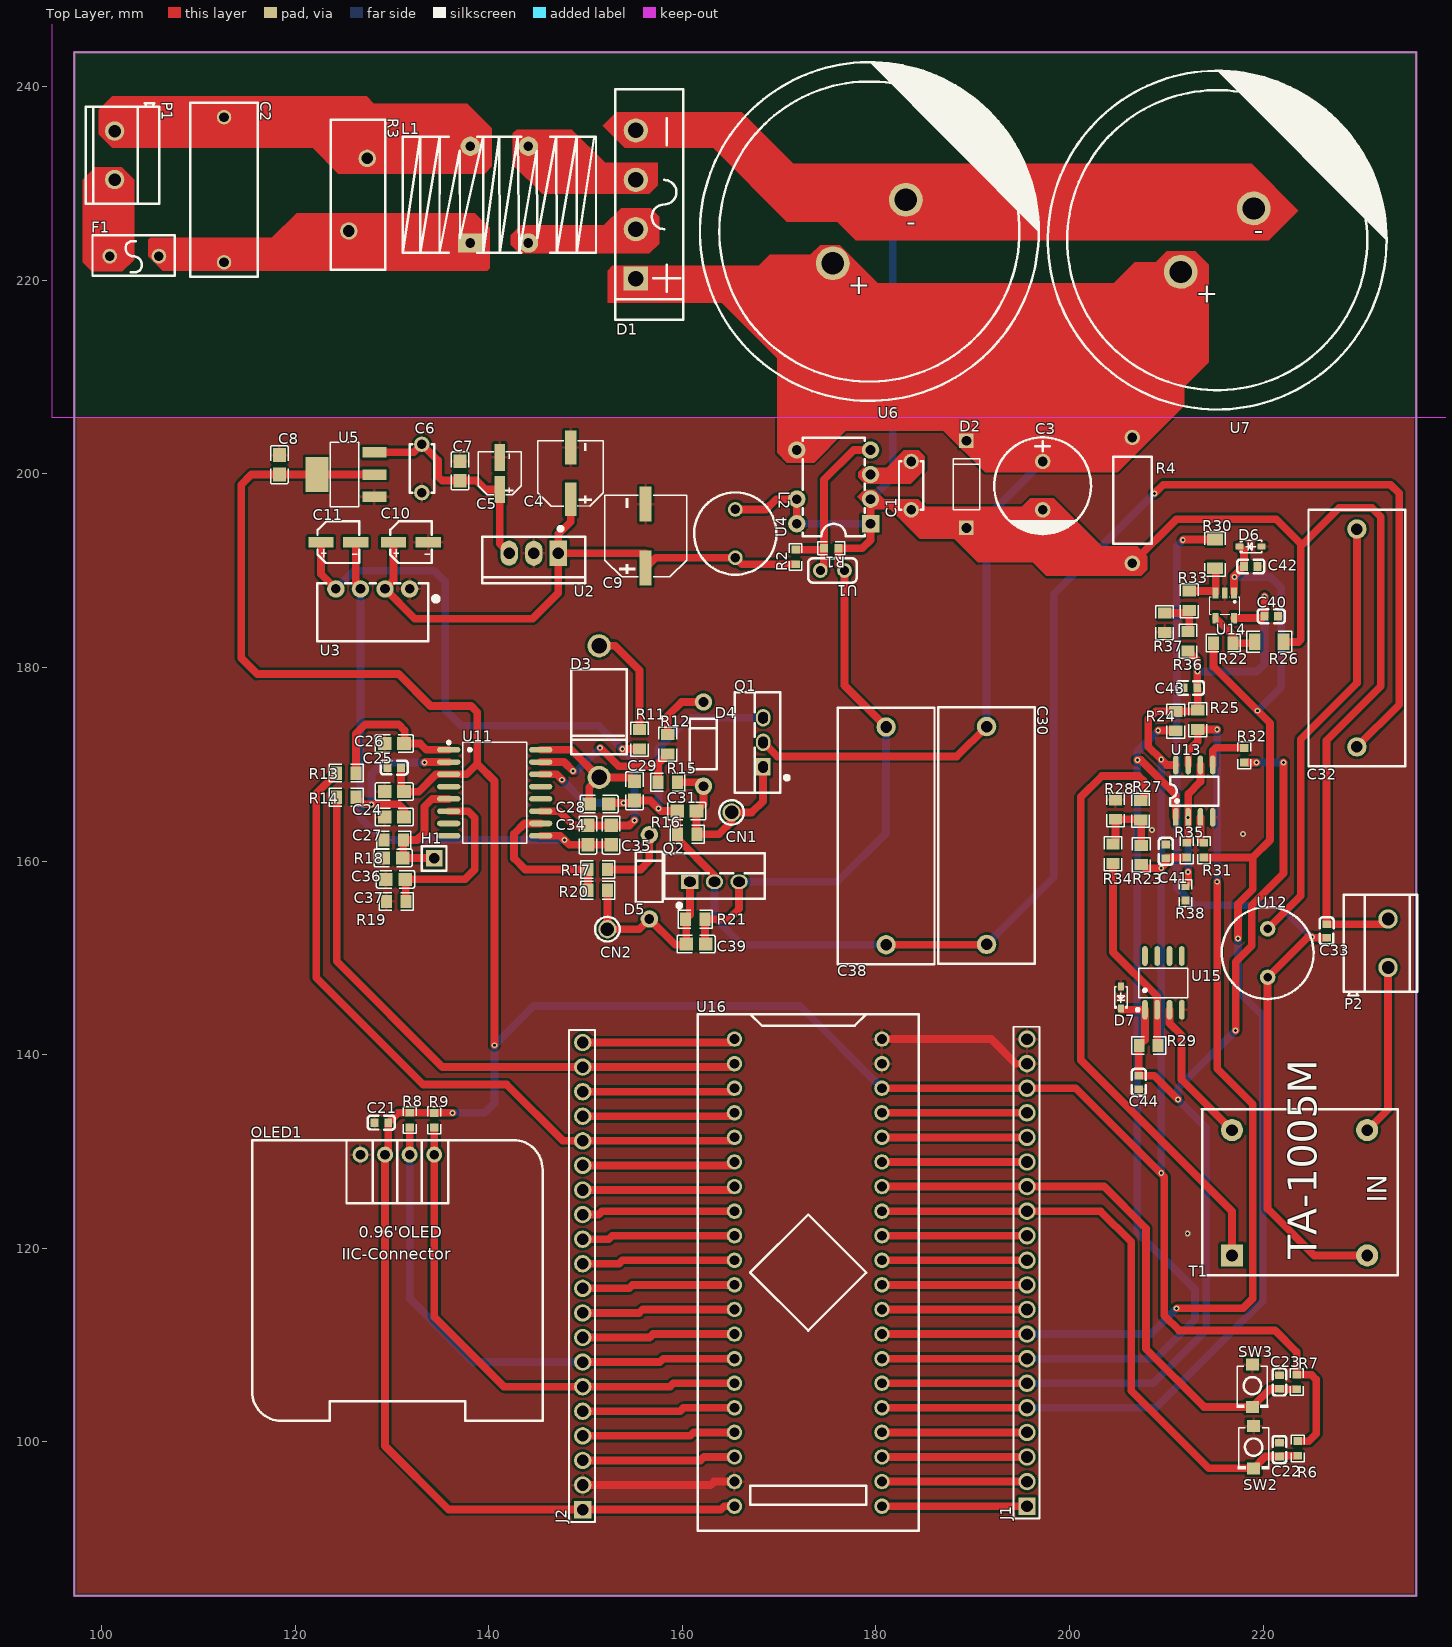
[diagram p0: Top Layer view]
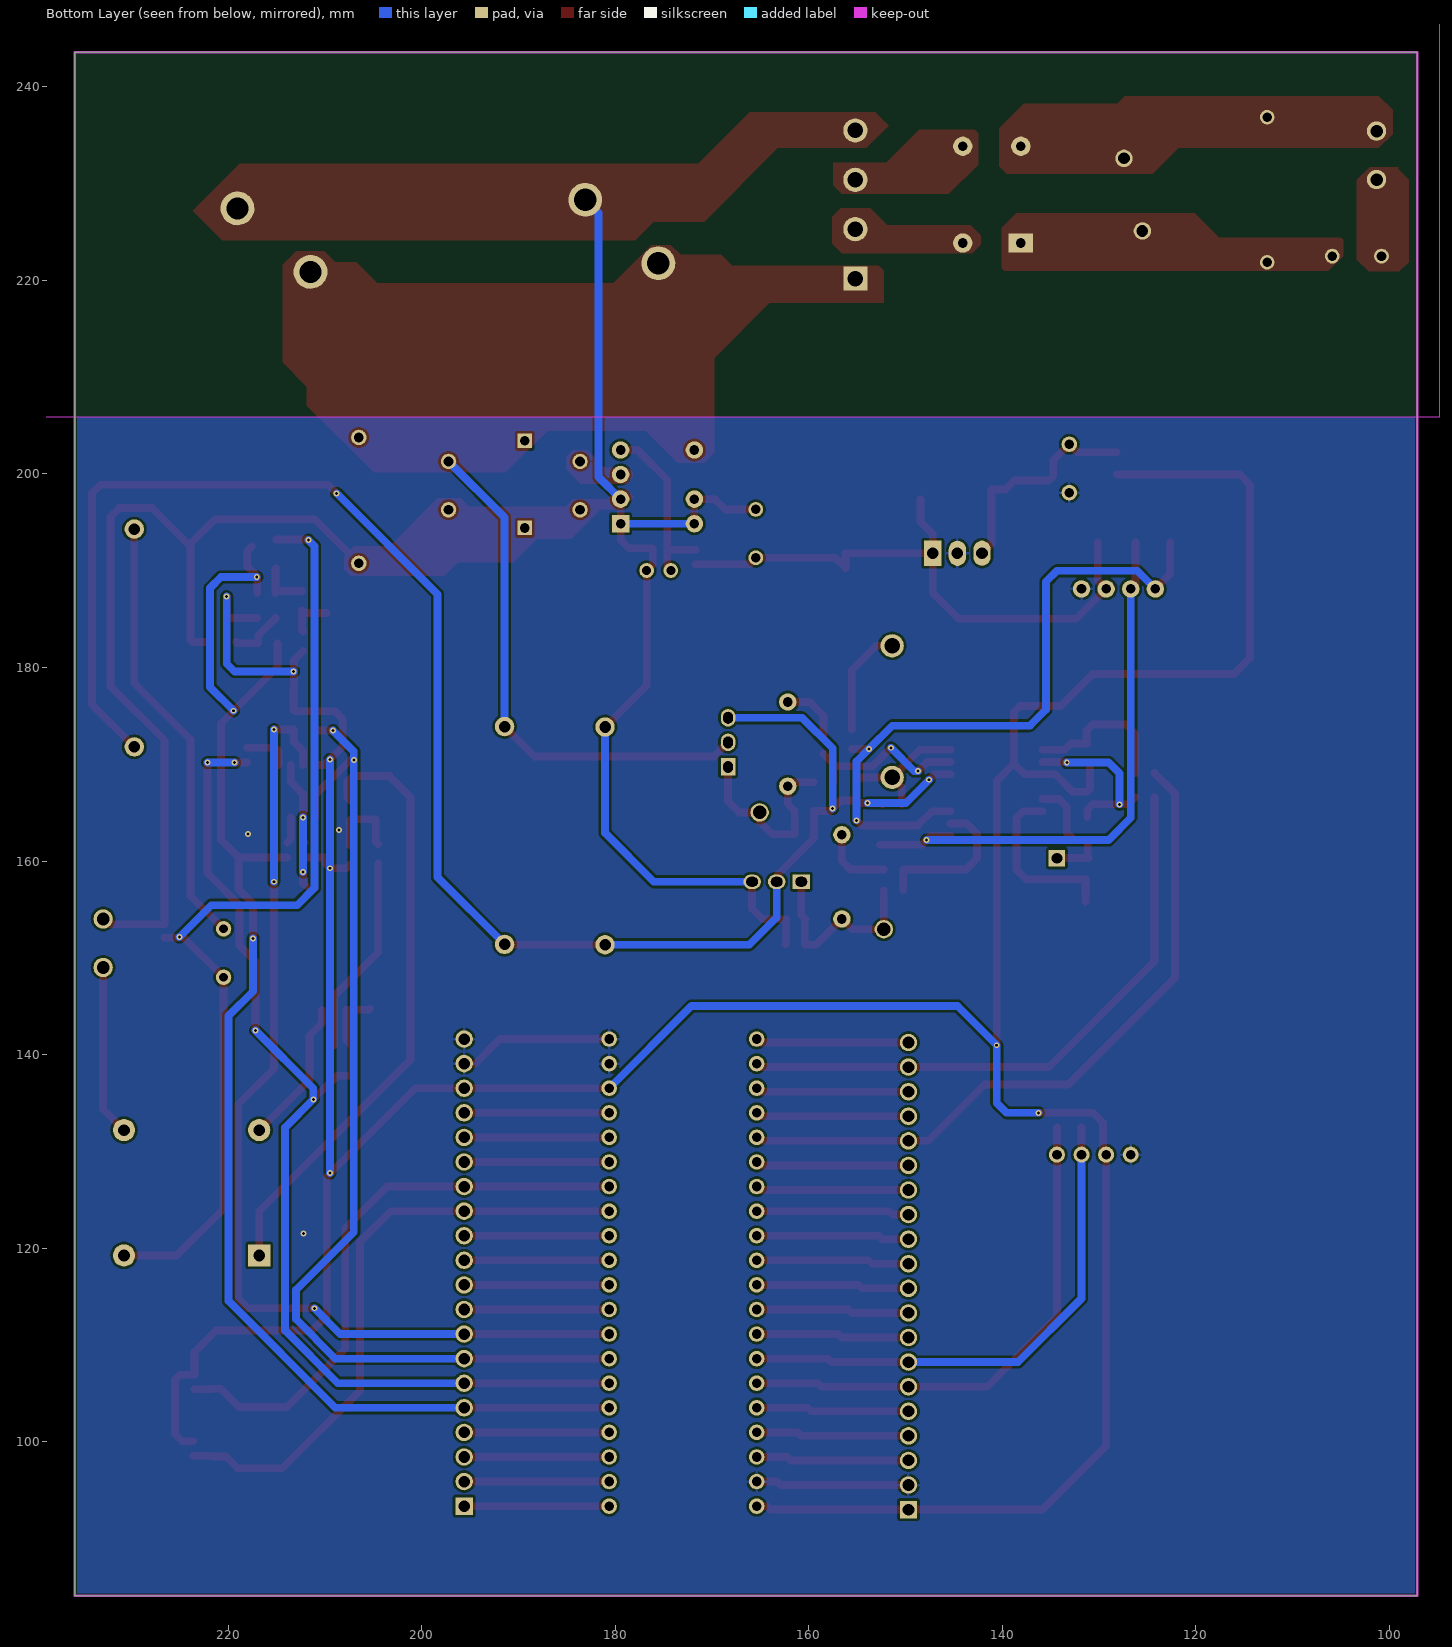
[diagram p1: Bottom Layer view, seen from below]
# Altium PCB MISC51807.pcbdoc
Units mm, origin at the board's own origin, x right, y up, seen from the top; angles counter-clockwise.
Board outline 138.68 x 159.51 mm, 2 copper layers (Top Layer, Bottom Layer), stack 1.58 mm thick; 107 components, 77 nets, 334 pads, 37 vias.

## Layer stack, top to bottom
Top Solder Mask Layer: solder mask 0.01, Dk 3.3
Top Layer: signal copper 0.035
Dielectric1: surface 1.51, FR4, Dk 4.5
Bottom Layer: signal copper 0.035
Bottom Solder Mask Layer: solder mask 0.01, Dk 3.3

## Board outline
97.155,243.586 97.155,84.074 235.839,84.074 235.839,243.586

## Design rules (kind name [scope] priority, off if disabled: settings)
BoardOutlineClearance copperThickness2oz_1 [All] p2 off: genericclearance=0.203 ignorepadtopadclearanceinfootprint=FALSE except(0: Arc-SplitContinuation Track-SplitContinuation SMDPad-SplitContinuation THPad-SplitContinuation Via-SplitContinuation Fill-SplitContinuation Region-SplitContinuation Poly-SplitContinuation Text-SplitContinuation Hole-SplitContinuation; 0.152: Arc-CutoutEdge SMDPad-CutoutEdge THPad-CutoutEdge Via-CutoutEdge Fill-CutoutEdge Region-CutoutEdge Text-CutoutEdge; 0.176: Hole-OutlineEdge Hole-CutoutEdge; 0.254: Poly-OutlineEdge Poly-CutoutEdge; 0.3: Arc-OutlineEdge Track-OutlineEdge SMDPad-OutlineEdge THPad-OutlineEdge Via-OutlineEdge Fill-OutlineEdge Region-OutlineEdge Text-OutlineEdge Track-CutoutEdge)
BoardOutlineClearance copperThickness1oz_1 [All] p4: genericclearance=0.102 ignorepadtopadclearanceinfootprint=FALSE except(0: Arc-SplitContinuation Track-SplitContinuation SMDPad-SplitContinuation THPad-SplitContinuation Via-SplitContinuation Fill-SplitContinuation Region-SplitContinuation Poly-SplitContinuation Text-SplitContinuation Hole-SplitContinuation; 0.152: SMDPad-CutoutEdge THPad-CutoutEdge Via-CutoutEdge Fill-CutoutEdge Region-CutoutEdge Text-CutoutEdge; 0.176: Hole-OutlineEdge Hole-CutoutEdge; 0.254: Poly-OutlineEdge Poly-CutoutEdge; 0.3: Arc-OutlineEdge Track-OutlineEdge SMDPad-OutlineEdge THPad-OutlineEdge Via-OutlineEdge Fill-OutlineEdge Region-OutlineEdge Text-OutlineEdge Arc-CutoutEdge Track-CutoutEdge)
Clearance copperThickness2oz [All] p1 off: gap=0.203 ignorepadtopadclearanceinfootprint=FALSE except(0.152: SMDPad-Track SMDPad-SMDPad THPad-Track SMDPad-THPad THPad-THPad Track-Via SMDPad-Via THPad-Via Via-Via Fill-Track Region-Track Fill-SMDPad Region-SMDPad Fill-THPad Region-THPad Fill-Via Region-Via Fill-Fill Fill-Region Region-Region Arc-Track Arc-SMDPad Arc-THPad Arc-Via Fill-Arc Region-Arc Arc-Arc Text-Track SMDPad-Text Text-THPad Text-Via Fill-Text Region-Text Arc-Text Text-Text; 0.176: Hole-Track Hole-SMDPad Hole-THPad Hole-Via Fill-Hole Region-Hole Hole-Arc Hole-Text; 0.254: Poly-Track Poly-SMDPad Poly-THPad Poly-Via Poly-Fill Poly-Region Poly-Poly Poly-Arc Poly-Text Poly-Hole)
Clearance copperThickness1oz [All] p3: gap=0.102 ignorepadtopadclearanceinfootprint=FALSE except(0.152: SMDPad-Track SMDPad-SMDPad THPad-Track SMDPad-THPad THPad-THPad Track-Via SMDPad-Via THPad-Via Via-Via Fill-Track Region-Track Fill-SMDPad Region-SMDPad Fill-THPad Region-THPad Fill-Via Region-Via Fill-Fill Fill-Region Region-Region Arc-Track Arc-SMDPad Arc-THPad Arc-Via Fill-Arc Region-Arc Arc-Arc Text-Track SMDPad-Text Text-THPad Text-Via Fill-Text Region-Text Arc-Text Text-Text; 0.176: Hole-Track Hole-SMDPad Hole-THPad Hole-Via Fill-Hole Region-Hole Hole-Arc Hole-Text; 0.254: Poly-Track Poly-SMDPad Poly-THPad Poly-Via Poly-Fill Poly-Region Poly-Poly Poly-Arc Poly-Text Poly-Hole)
DiffPairsRouting differentialPair [All] p1: maxlimit=0.152 minlimit=0.152 mostfreqgap=0.152 toplayer_minwidth=0.127 toplayer_prefwidth=0.254 toplayer_maxwidth=2.54 toplayer_mingap=0.152 toplayer_prefgap=0.152 toplayer_maxgap=0.152 bottomlayer_minwidth=0.127 bottomlayer_prefwidth=0.254 bottomlayer_maxwidth=2.54 bottomlayer_mingap=0.152 bottomlayer_prefgap=0.152 bottomlayer_maxgap=0.152 maxuncoupledlength=0.254
HoleToHoleClearance otherClearance [All] p1: gap=0.3 allowstackedmicrovias=TRUE
Length netLength [All] p1: minlimit=0 maxlimit=0
MatchedLengths netLengthTolerance [All] p1: tolerance=25.4
PasteMaskExpansion pasteMaskExpansion [All] p1: expansion=0
PlaneConnect innerPlane [All] p1: planeconnectstyle=Relief reliefexpansion=0.508 reliefentries=4 reliefconductorwidth=0.254 reliefairgap=0.254
PolygonConnect copperRegion [(InNet('GND'))] p1: connectstyle=Relief reliefconductorwidth=0.254 reliefentries=4 polygonreliefangle="90 Angle" airgapwidth=0.254 via.connectstyle=Relief via.reliefconductorwidth=0.254 via.reliefentries=4 via.polygonreliefangle="90 Angle" via.airgapwidth=0.254
RoutingVias viaSize [All] p1: holewidth=0.305 width=0.61 viastyle="Through Hole" minholewidth=0.3 minwidth=0.5 maxholewidth=6.3 maxwidth=10
SolderMaskExpansion solderMaskExpansion [IsVia] p1: expansion=-25.4 istentingtop=TRUE
SolderMaskExpansion solderMaskExpansion [All] p2: expansion=0.051 istentingtop=FALSE
Width copperThickness2oz_2 [All] p1 off: maxlimit=2.54 minlimit=0.203 preferedwidth=0.254
Width copperThickness1oz_2 [All] p2: maxlimit=2.54 minlimit=0.127 preferedwidth=0.254

## Components (designator, comment, footprint, x,y, rotation, side; value= is the part's Value field where it differs from the comment)
C1 "100nF" CAP-TH_L5.0-W2.5-P5.00-D1.0 183.639,198.789 r90 top
C2 "330nF" CAP-TH_L18.0-W7.0-P15.00-D0.7 112.649,229.362 r270 top
C3 "10uF" CAP-TH_BD10.0-P5.00-D0.6-FD_1 197.228,198.789 r270 top
C4 "100uF" CAP-SMD_BD6.3-L6.6-W6.6-FD 148.46,200.059 r90 top
C5 "10uF" CAP-SMD_BD4.0-L4.3-W4.3-FD 141.13,200.044 r90 top
C6 "100nF" CAP-TH_L5.0-W2.5-P5.00-D1.0 133.093,200.567 r90 top
C7 "10uF" C0805 137.03,200.313 r270 top
C8 "10uF" C0805 118.361,200.948 r270 top
C9 "470uF" CAP-SMD_BD8.0-L8.3-W8.3-LS9.2-FD-H10.5 156.207,193.582 r90 top
C10 "10uF" CAP-SMD_BD4.0-L4.3-W4.3-FD_1 131.95,192.947 r0 top
C11 "10uF" CAP-SMD_BD4.0-L4.3-W4.3-FD_1 124.457,192.947 r0 top
C21 "100nF" C0603 128.905,132.969 r0 top
C22 "100nF" C0603 221.692,99.187 r270 top
C23 "100nF" C0603 221.692,106.172 r270 top
C24 "10uF" C0805 130.238,167.171 r0 top
C25 "100nF" C0603 130.245,169.652 r0 top
C26 "22PF" C0805 130.238,172.137 r180 top
C27 "22PF" C0805 130.238,164.548 r0 top
C28 "100nf" C0805 151.395,165.883 r0 top
C29 "2.2uf" C0805 155.067,167.259 r270 top
C30 "10uF/630V CBB" "1uf/630V CBB" 191.389,162.687 r270 top
C31 "1nf" C0805 160.463,165.162 r0 top
C32 "10uF/630V CBB" "1uf/630V CBB" 229.743,183.007 r90 top
C33 "100nF" C0603 226.568,152.781 r270 top
C34 "100nF" C0805 150.241,162.687 r270 top
C35 "2.2uf" C0805 152.654,162.687 r270 top
C36 "22pf" C0805 130.111,160.326 r0 top
C37 "100nF" C0805 130.365,158.115 r0 top
C38 "10uF/630V CBB" "1uf/630V CBB" 181.102,162.56 r90 top
C39 "1nf" C0805 161.415,151.421 r180 top
C40 "100nF" C0603 220.853,185.293 r0 top
C41 "100nF" C0603 209.955,161.004 r90 top
C42 "100nF" C0603 218.726,190.442 r180 top
C43 "100nF" C0603 212.495,177.895 r180 top
C44 "100nF" C0603 207.161,137.128 r270 top
CN1 "RH-5001" TEST-TH_BD2.54-P1.4_BLACK 165.083,165.025 r0 top
CN2 "RH-5001" TEST-TH_BD2.54-P1.4_BLACK 152.256,152.96 r0 top
D1 "KBU810" DIO-BG-TH_L23.2-W6.8-P5.10_KBU 155.194,227.838 r270 top
D2 "BYV26C" DO-41_BD2.6-L5.1-P9.00-D0.8-RD 189.354,198.916 r270 top
D3 "SR5100" DO-201AD_BD5.3-L8.4-P12.50-D1.4-RD 151.395,175.439 r90 top
D4 "1N5819" DO-41_BD2.4-L4.7-P8.70-D0.9-FD 162.179,172.085 r90 top
D5 "1N5819" DO-41_BD2.4-L4.7-P8.70-D0.9-FD 156.591,158.369 r90 top
D6 "BZT52C3V3S" SOD-323_L1.7-W1.3-LS2.6-RD 218.718,192.5 r0 top
D7 "BZT52C3V3S" SOD-323_L1.7-W1.3-LS2.6-RD 205.312,145.894 r90 top
F1 "MTS1315A" FUSE-TH_L8.4-W4.0-P5.08-D0.6 103.378,222.504 r0 top
H1 "PZ254V-11-01P" HDR-TH_1P-P2.54-V-M 134.366,160.274 r0 top
J1 "2.54-1*20P直针" HDR-TH_20P-P2.54-V-M-1 195.612,117.48 r90 top
J2 "2.54-1*20P直针" HDR-TH_20P-P2.54-V-M-1 149.708,117.122 r90 top
L1 "PDMCAT16128-103ML" IND-TH_4P-L20.0-W12.0-P6.00-LS10.0-BL 141.097,228.854 r0 top
L2 "1mH" IND-TH_BD8.5-P5.00-D0.6 165.478,193.836 r270 top
OLED1 "" 0.96OLED_4P 130.556,129.667 r0 top
P1 "CONN-TH_2P-P5.00" CONN-TH_2P-P5.00 101.346,232.918 r270 top
P2 "CONN-TH_2P-P5.00" CONN-TH_2P-P5.00 232.918,151.511 r90 top
Q1 "IRF840" TO-220-3_L10.2-W4.5-P2.54-L-1 168.348,172.264 r90 top
Q2 "IRF840" TO-220-3_L10.2-W4.5-P2.54-L-1 163.322,157.861 r0 top
R1 "6.2kΩ" R0603 175.384,192.312 r180 top
R2 "20kΩ" R0603 171.701,191.423 r90 top
R3 "420pF@1kHz" RES-TH_L15.5-W5.6-P7.50-D0.8-S1.90 126.492,228.854 r270 top
R4 "220kΩ" RES-TH_BD3.9-L9.0-P13.00-D0.8 206.499,197.265 r90 top
R6 "10kΩ" R0603_1 223.597,99.314 r90 top
R7 "10kΩ" R0603_1 223.47,106.172 r90 top
R8 "4.7kΩ" R0603 131.826,133.24 r90 top
R9 "4.7kΩ" R0603 134.366,133.223 r90 top
R11 "4.7R" R0805#1 155.575,172.593 r90 top
R12 "4.7R" R0805#1 158.496,172.085 r90 top
R13 "47R" R0805#1 125.285,169.089 r0 top
R14 "47R" R0805#1 125.285,166.603 r0 top
R15 "10r" R0805#1 158.496,168.148 r180 top
R16 "10K" R0805#1 160.515,162.766 r0 top
R17 "4.7R" R0805#1 151.257,159.131 r0 top
R18 "10K" R0805#1 130.175,162.179 r0 top
R19 "4.7k" R0805#1 130.429,155.829 r0 top
R20 "10r" R0805#1 151.257,156.972 r180 top
R21 "10K" R0805#1 161.341,153.978 r180 top
R22 "10kΩ" R0805#1 215.89,182.518 r180 top
R23 "10kΩ" R0805#1 207.415,160.623 r90 top
R24 "10kΩ" R0805#1 210.971,174.466 r270 top
R25 "10kΩ" R0805#1 213.257,174.593 r270 top
R26 "1MΩ" R1206 220.634,182.645 r180 top
R27 "100Ω" R0805#1 207.352,165.259 r270 top
R28 "10kΩ" R0805#1 204.748,165.322 r90 top
R29 "820Ω" R0805#2 208.177,140.938 r0 top
R30 "1MΩ" R1206 215.035,191.738 r270 top
R31 "1kΩ" R0603 213.892,161.131 r90 top
R32 "1kΩ" R0603 218.059,170.942 r270 top
R33 "10kΩ" R0805#1 212.368,186.912 r90 top
R34 "100Ω" R0805#1 204.494,160.75 r90 top
R35 "100kΩ" R0603 212.114,161.131 r270 top
R36 "10kΩ" R0805#1 212.241,182.721 r270 top
R37 "10kΩ" R0805#1 209.828,184.626 r90 top
R38 "3.3kΩ" R0603_NEW 211.987,156.686 r90 top
SW2 "TS-1088-AR02016" SW-SMD_L3.9-W3.0-P4.45 219.025,99.441 r270 top
SW3 "TS-1088-AR02016" SW-SMD_L3.9-W3.0-P4.45 218.898,105.791 r270 top
T1 "TA-1005M" TA-1005M 216.789,119.253 r90 top
U1 "10nF" CAP-TH_L5.0-W2.5-P2.50-D0.5 175.511,190.026 r180 top
U2 "LM7805" TO-220-3_L10.0-W4.5-P2.54-L 144.65,191.804 r180 top
U3 "260kHz" PWRM-TH_4P-L11.5-W6.0-P2.54_B1503S 128.013,188.121 r180 top
U4 "LNK304PN" DIP-8_7P-L9.7-W6.4-P2.54-LS7.6-BL-PE6 175.638,198.662 r90 top
U5 "AMS1117-3.3" SOT-223-3_L6.5-W3.4-P2.30-LS7.0-BR 125.219,199.932 r0 top
U6 "470uF" CAP-TH_BD35.0-P10.00-D1.5-FD 179.324,225.044 r0 top
U7 "470uF" CAP-TH_BD35.0-P10.00-D1.5-FD 215.265,224.155 r0 top
U11 "UCC21520ADWR" SOIC-16_L10.3-W7.5-P1.27-LS10.3-BL 140.618,167.057 r270 top
U12 "2.5mH" IND-TH_BD9.5-P5.00-D0.7 220.472,150.495 r270 top
U13 "LM393DR" SOIC-8_L5.0-W4.0-P1.27-LS6.0-BL 212.896,167.227 r0 top
U14 "AD8605ARTZ-REEL7" SOT-23-5_L3.0-W1.7-P0.95-LS2.8-BR 216.051,186.404 r90 top
U15 "LM358DT" SOIC-8_L4.9-W3.9-P1.27-LS6.0-BL 209.701,147.415 r0 top
U16 "STM32F103C8T6-Card" CONN-TH_L53.3-W22.9_STM32F103C8T6-CARD 173.006,117.48 r270 top

## Footprints (in the part's own frame and the unit in brackets; to place one, negate y for a bottom-side part, rotate by r counter-clockwise, add the part's x,y. Pads: shape width x height; smd on the part's side, far side on the other; paste and mask are expansions set on the pad)
0.96OLED_4P [mm]
  round 1.65 hole 1 copper offset 0,0: 1(-3.81,-0.001) 2(-1.27,0.002) 3(1.27,0.002) 4(3.81,0.002)
  silkscreen extent -15,-27.5 15,1.5
"1uf/630V CBB" [mm]
  round 2 hole 1.2: 1(-11.208,0.047) 2(11.292,0.047)
  silkscreen extent -13.21,-4.95 13.29,5.05
C0603 [mm]
  rect 0.8x0.9 smd paste+0 mask+0.051: 1(-0.7,0) 2(0.7,0)
  silkscreen extent -1.41,-0.71 1.39,0.72
C0805 [mm]
  rect 1.41x1.35 smd paste-100 mask+0.051: 1(-1,0) 2(1,0)
  silkscreen extent -1.96,-0.9 1.96,0.9
CAP-SMD_BD4.0-L4.3-W4.3-FD [mm]
  rect 2.8x1.1 smd: 1(-1.661,0) 2(1.661,0)
  silkscreen extent -2.22,-2.23 2.24,2.23
CAP-SMD_BD4.0-L4.3-W4.3-FD_1 [mm]
  rect 2.6x1.1 smd: 1(-1.8,0) 2(1.8,0)
  silkscreen extent -2.15,-2.15 2.15,2.15
CAP-SMD_BD6.3-L6.6-W6.6-FD [mm]
  rect 3.5x1.2 smd: 1(-2.67,0) 2(2.67,0)
  silkscreen extent -3.38,-3.38 3.38,3.38
CAP-SMD_BD8.0-L8.3-W8.3-LS9.2-FD-H10.5 [mm]
  rect 3.61x1.26 smd: 1(-3.295,0) 2(3.295,0)
  silkscreen extent -4.23,-4.23 4.23,4.23
CAP-TH_BD10.0-P5.00-D0.6-FD_1 [mm]
  round 1.6 hole 1 paste+0 mask+0.05: 1(-2.5,0) 2(2.5,0)
  silkscreen extent -5,-5 5.08,5
CAP-TH_BD35.0-P10.00-D1.5-FD [mm]
  round 3.5 hole 2.3: 1(-3.774,-3.28) 2(3.774,3.28)
  silkscreen extent -17.5,-17.5 17.5,17.5
CAP-TH_L5.0-W2.5-P2.50-D0.5 [mil]
  round 60 hole 36 paste+0 mask+1.97: 1(-49.21,0) 2(49.21,0)
  silkscreen extent -98,-49 98,49
CAP-TH_L5.0-W2.5-P5.00-D1.0 [mm]
  round 1.6 hole 1: 1(-2.5,0) 2(2.5,0)
  silkscreen extent -2.5,-1.27 2.5,1.25
CAP-TH_L18.0-W7.0-P15.00-D0.7 [mm]
  round 1.5 hole 1: 1(-7.5,0) 2(7.5,0)
  silkscreen extent -9,-3.5 9,3.5
CONN-TH_2P-P5.00 [mm]
  round 2 hole 1.3: 1(-2.504,0) 2(2.504,0)
  silkscreen extent -5.4,-3 5,4.6
CONN-TH_L53.3-W22.9_STM32F103C8T6-CARD [mm]
  round 1.6 hole 1: 1(-24.13,-7.62) 2(-21.59,-7.62) 3(-19.05,-7.62) 4(-16.51,-7.62) 5(-13.97,-7.62) 6(-11.43,-7.62) 7(-8.89,-7.62) 8(-6.35,-7.62) 9(-3.81,-7.62) 10(-1.27,-7.62) 11(1.27,-7.62) 12(3.81,-7.62) 13(6.35,-7.62) 14(8.89,-7.62) 15(11.43,-7.62) 16(13.97,-7.62) 17(16.51,-7.62) 18(19.05,-7.62) 19(21.59,-7.62) 20(24.13,-7.62) 21(24.13,7.62) 22(21.59,7.62) 23(19.05,7.62) 24(16.51,7.62) 25(13.97,7.62) 26(11.43,7.62) 27(8.89,7.62) 28(6.35,7.62) 29(3.81,7.62) 30(1.27,7.62) 31(-1.27,7.62) 32(-3.81,7.62) 33(-6.35,7.62) 34(-8.89,7.62) 35(-11.43,7.62) 36(-13.97,7.62) 37(-16.51,7.62) 38(-19.05,7.62) 39(-21.59,7.62) 40(-24.13,7.62)
  silkscreen extent -26.67,-11.43 26.67,11.43
DIO-BG-TH_L23.2-W6.8-P5.10_KBU [mm]
  rect 2.5x2.5 hole 1.6: 1(7.65,0)
  round 2.5 hole 1.6: 2(2.55,0) 3(-2.55,0) 4(-7.65,0)
  silkscreen extent -11.9,-2.1 11.9,4.9
DIP-8_7P-L9.7-W6.4-P2.54-LS7.6-BL-PE6 [mm]
  rect 1.8x1.8 hole 1: 1(-3.81,-3.81)
  round 1.8 hole 1: 2(-1.27,-3.81) 3(1.27,-3.81) 4(3.81,-3.81) 5(3.81,3.81) 7(-1.27,3.81) 8(-3.81,3.81)
  silkscreen extent -5.08,-3.2 5.08,3.2
DO-41_BD2.4-L4.7-P8.70-D0.9-FD [mm]
  round 1.8 hole 1: 1(-4.35,0) 2(4.35,0)
  silkscreen extent -2.6,-1.4 2.6,1.4
DO-41_BD2.6-L5.1-P9.00-D0.8-RD [mm]
  rect 1.5x1.5 hole 1: 1(-4.5,0) 2(4.5,0)
  silkscreen extent -2.63,-1.38 2.63,1.38
DO-201AD_BD5.3-L8.4-P12.50-D1.4-RD [mm]
  round 2.4 hole 1.6: 1(-6.8,0) 2(6.8,0)
  silkscreen extent -4.4,-2.85 4.4,2.85
FUSE-TH_L8.4-W4.0-P5.08-D0.6 [mil]
  round 60 hole 39.37 paste+0 mask+1.97: 1(-100,0) 2(100,0)
  silkscreen extent -170,-80 165,85
HDR-TH_1P-P2.54-V-M [mm]
  rect 1.7x1.7 hole 1.1: 1(0,0)
  silkscreen extent -1.27,-1.27 1.27,1.27
HDR-TH_20P-P2.54-V-M-1 [mm]
  rect 1.8x1.8 hole 1.2 paste+0 mask+0.051: 1(-24.13,0)
  round 1.8 hole 1.2 paste+0 mask+0.051: 2(-21.59,0) 3(-19.05,0) 4(-16.51,0) 5(-13.97,0) 6(-11.43,0) 7(-8.89,0) 8(-6.35,0) 9(-3.81,0) 10(-1.27,0) 11(1.27,0) 12(3.81,0) 13(6.35,0) 14(8.89,0) 15(11.43,0) 16(13.97,0) 17(16.51,0) 18(19.05,0) 19(21.59,0) 20(24.13,0)
  silkscreen extent -25.4,-1.27 25.4,1.4
IND-TH_4P-L20.0-W12.0-P6.00-LS10.0-BL [mm]
  rect 2.5x2 hole 1 copper offset 0,0 paste+0 mask+0.05: 1(-3,-5)
  round 2 hole 1 paste+0 mask+0.05: 2(-3,5)
  round 2 hole 1 copper offset 0,0 paste+0 mask+0.05: 3(3,5) 4(3,-5)
  silkscreen extent -10,-6 9.98,6
IND-TH_BD8.5-P5.00-D0.6 [mil]
  round 60 hole 39.37: 1(-98.43,0) 2(98.42,0)
  silkscreen extent -167,-167 167,167
IND-TH_BD9.5-P5.00-D0.7 [mm]
  round 1.6 hole 0.9: 1(-2.5,0) 2(2.5,0)
  silkscreen extent -4.75,-4.75 4.75,4.75
PWRM-TH_4P-L11.5-W6.0-P2.54_B1503S [mm]
  round 1.8 hole 1 paste+0 mask+0.05: 1(-3.81,0) 2(-1.27,0) 3(1.27,0) 4(3.81,0)
  silkscreen extent -6.77,-0.59 5.75,5.43
R0603 [mm]
  rect 0.806x0.864 smd paste-100 mask+0.051: 1(-0.753,0) 2(0.753,0)
  silkscreen extent -1.39,-0.66 1.39,0.66
R0603_1 [mm]
  rect 0.806x0.864 smd paste-100 mask+0.051: 1(-0.753,0) 2(0.753,0)
  silkscreen extent -1.39,-0.66 1.39,0.66
R0603_NEW [mm]
  rect 0.806x0.864 smd paste-100 mask+0.051: 1(-0.753,0) 2(0.753,0)
  silkscreen extent -1.39,-0.66 1.39,0.66
R0805#1 [mm]
  rect 1.133x1.377 smd paste-100 mask+0.051: 1(-1,0) 2(1,0)
  silkscreen extent -1.76,-0.92 1.76,0.92
R0805#2 [mm]
  rect 1.133x1.377 smd paste-100 mask+0.051: 1(-0.966,0) 2(0.966,0)
  silkscreen extent -1.76,-0.92 1.76,0.92
R1206 [mm]
  rect 1.208x1.701 smd paste-100 mask+0.051: 1(-1.479,0) 2(1.479,0)
  silkscreen extent -2.31,-1.08 2.31,1.08
RES-TH_BD3.9-L9.0-P13.00-D0.8 [mm]
  round 1.6 hole 1 paste+0 mask+0.05: 1(-6.5,0) 2(6.5,0)
  silkscreen extent -4.5,-2 4.5,2
RES-TH_L15.5-W5.6-P7.50-D0.8-S1.90 [mm]
  round 1.8 hole 1.2 paste+0 mask+0.05: 1(-3.75,0.95) 2(3.75,-0.95)
  silkscreen extent -7.75,-2.8 7.75,2.8
SOD-323_L1.7-W1.3-LS2.6-RD [mm]
  rect 0.83x0.63 smd paste+0 mask+0.05: 1(-1.14,0) 2(1.14,0)
  silkscreen extent -1.08,-0.64 1.13,0.64
SOIC-8_L4.9-W3.9-P1.27-LS6.0-BL [mm]
  oval 0.588x2.045 smd: 1(-1.905,-2.772) 2(-0.635,-2.772) 3(0.635,-2.772) 4(1.905,-2.772) 5(1.905,2.772) 6(0.635,2.772) 7(-0.635,2.772) 8(-1.905,2.772)
  silkscreen extent -2.8,-2.92 2.53,1.52
SOIC-8_L5.0-W4.0-P1.27-LS6.0-BL [mil]
  oval 22.38x76.78 smd: 1(-75,-106.5) 2(-25,-106.5) 3(25,-106.5) 4(75,-106.5) 5(75,106.5) 6(25,106.5) 7(-25,106.5) 8(-75,106.5)
  silkscreen extent -98,-59 98,59
SOIC-16_L10.3-W7.5-P1.27-LS10.3-BL [mm]
  oval 0.574x2.401 smd: 1(-4.445,-4.75) 2(-3.175,-4.75) 3(-1.905,-4.75) 4(-0.635,-4.75) 5(0.635,-4.75) 6(1.905,-4.75) 7(3.175,-4.75) 8(4.445,-4.75) 9(4.445,4.75) 10(3.175,4.75) 11(1.905,4.75) 12(0.635,4.75) 13(-0.635,4.75) 14(-1.905,4.75) 15(-3.175,4.75) 16(-4.445,4.75)
  silkscreen extent -5.33,-4.9 5.23,3.32
SOT-23-5_L3.0-W1.7-P0.95-LS2.8-BR [mm]
  rect 1.1x0.6 smd: 1(1.3,-0.95) 2(1.3,0) 3(1.3,0.95) 4(-1.3,0.95) 5(-1.3,-0.95)
  silkscreen extent -0.9,-1.55 0.9,1.55
SOT-223-3_L6.5-W3.4-P2.30-LS7.0-BR [mm]
  rect 2.5x1.1 smd: 1(2.97,-2.3) 2(2.97,0) 3(2.97,2.3)
  rect 2.34x3.6 smd: 4(-2.97,0)
  silkscreen extent -1.57,-3.33 1.37,3.33
SW-SMD_L3.9-W3.0-P4.45 [mm]
  rect 1.23x1.36 smd: 1(-2.185,0) 2(2.185,0)
  silkscreen extent -2.03,-1.62 2.25,1.62
TA-1005M [mil]
  round 90 hole 47.25 paste+0 mask+2: 1(0,-550) 2(510,-550) 3(510,0)
  rect 90x90 hole 48.25 paste+0 mask+2: 4(0,0)
  silkscreen extent -80,-675 596,123
TEST-TH_BD2.54-P1.4_BLACK [mm]
  round 1.9 hole 1.39: 1(0,0)
  silkscreen extent -1.27,-1.27 1.27,1.27
TO-220-3_L10.0-W4.5-P2.54-L [mm]
  rect 1.8x2.6 hole 1.2: 1(-2.54,0.005)
  oval 1.8x2.6 hole 1.2: 2(0,0.005)
  oval 1.8x2.6 hole 1.2 copper offset 0,0: 3(2.54,-0.005)
  silkscreen extent -5.3,-2.73 5.3,3.09
TO-220-3_L10.2-W4.5-P2.54-L-1 [mm]
  rect 1.8x1.5 hole 1 slot 1.2 at 0 deg: 1(-2.54,0)
  oval 1.8x1.5 hole 1 slot 1.2 at 0 deg: 2(0,0) 3(2.54,0)
  silkscreen extent -5.2,-2.65 5.2,2.95

## Via types
v1: diameter 0.61, hole 0.305, Top Layer to Bottom Layer, 37 vias

## Nets (pads, with @x,y where several pads share a name; then routed paths per layer and width w, separated by ;. In a path a pad name is that pad's centre, name@x,y a point inside that pad or via, vN(x,y) a via of type N, cw(c..) or ccw(c..) an arc to the next point about the centre after c; other vN are vias at no path point)
3.3V: U11.8
3V3: C8.2 C21.2 C24.2 C25.2 C40.1 C41.1 C43.1 J1.18 J2.1 OLED1.2 R6.2 R7.2 R8.2 R9.2 R23.1 R24.1 R25.1 R35.2 R36.2 U5.2 U5.4 U11.3 U13.8 U14.5 U16.20 U16.38 | length 402.2
  Top Layer w0.8: U5.2 U5.4 118.377,199.932 C8.2 115.493,199.948 114.427,198.882 114.427,180.975 116.078,179.324 130.683,179.324 133.985,176.022 138.176,176.022 138.811,175.387 138.811,170.053 ; C25.2 130.945,167.464 C24.2 132.754,167.171 134.545,168.962 U11.3 137.72,168.962 138.811,170.053 ; v1(136.271,133.985) 131.835,133.985 R8.2 130.63,133.994 C21.2 129.605,129.987 129.286,129.668 129.286,99.568 135.862,92.992 J2.1 163.975,92.992 164.332,93.35 U16.20 ; v1(140.589,140.97) 140.589,168.275 138.811,170.053 ; U16.38 J1.18 200.655,136.53 v1@209.431,127.754 ; R23.1 207.78,159.258 209.423,159.258 209.955,159.79 C41.1 210.029,160.378 R35.2 ; v1(209.481,127.762) 209.473,127.754 v1@209.431,127.754 ; U13.8 210.052,169.932 v1(209.481,170.503) 208.153,171.831 208.153,174.666 208.953,175.466 R24.1 213.13,175.466 R25.1 213.257,177.833 C43.1 213.195,180.767 R36.2 ; U14.5 219.964,185.104 C40.1 v1(220.153,187.325) ; R6.2 224.731,100.067 225.502,100.838 225.502,106.426 225.003,106.925 R7.2 223.47,109.27 221.234,111.506 211.328,111.506 209.804,113.03 209.804,127.381 v1@209.431,127.754
  Bottom Layer w0.8: v1(136.271,133.985) 139.573,133.985 140.589,135.001 v1(140.589,140.97) 144.653,145.034 172.122,145.034 U16.38 ; v1(209.481,127.762) v1(209.481,159.258) v1(209.481,170.503) ; v1(213.233,179.578) 219.329,179.578 220.153,180.402 v1(220.153,187.325)
$1N282: D3.2 R11.2 | length 11.3
  Top Layer w0.8: D3.2 153.04,182.24 155.575,179.705 R11.2
$1N289: D5.2 R17.2 | length 7.4
  Top Layer w0.8: R17.2 155.702,159.131 156.591,160.02 D5.2
$1N290: R12.1 R15.2 U11.15 | length 17.7
  Top Layer w0.8: U11.15 147.776,170.232 v1(148.717,169.291) ; v1(151.511,171.704) 153.429,169.786 157.496,169.786 ; R15.2 157.496,169.786 ; R12.1 157.496,170.085 157.496,169.786
  Bottom Layer w0.8: v1(148.717,169.291) 149.098,169.291 v1(151.511,171.704)
$1N291: D4.2 R12.2 | length 6.2
  Top Layer w0.8: R12.2 158.496,175.006 159.925,176.435 D4.2
$1N295: C31.2 CN1.1 D4.1 Q1.1 R15.1 R16.2 | length 20.5
  Top Layer w0.8: R15.1 161.766,168.148 D4.1 162.179,165.878 C31.2 161.463,162.818 R16.2 163.782,162.766 165.083,164.067 CN1.1 167.184,165.025 168.348,166.189 Q1.1
$1N299: R17.1 R20.2 U11.10 | length 16
  Top Layer w0.8: U11.10 143.689,163.882 142.621,162.814 142.621,160.274 143.764,159.131 R17.1 R20.2
$1N304: C28.1 C29.1 D3.1 U11.16 | length 14.2
  Top Layer w0.8: U11.16 148.532,171.502 D3.1 ; C28.1 150.395,167.639 D3.1 ; C29.1 154.687,168.639 D3.1
$1N305: C36.2 H1.1 R18.2 U11.5 | length 13.2
  Top Layer w0.8: H1.1 134.314,160.326 C36.2 131.175,160.391 R18.2 132.588,162.179 133.35,162.941 133.35,165.608 134.164,166.422 U11.5
$1N312: C27.2 R14.2 U11.2 | length 17.9
  Top Layer w0.8: R14.2 127.026,165.862 v1(127.896,165.862) 130.683,165.862 131.238,165.307 C27.2 ; v1(133.35,170.18) 133.402,170.232 U11.2
  Bottom Layer w0.8: v1(127.896,165.862) 127.896,169.044 129.032,170.18 v1(133.35,170.18)
$1N313: C26.1 R13.2 U11.1 | length 16
  Top Layer w0.8: R13.2 126.285,173.148 127.254,174.117 130.683,174.117 131.318,173.482 131.318,172.218 C26.1 132.917,172.137 133.552,171.502 U11.1
$1N314: C37.2 R19.2 U11.6 | length 18.2
  Top Layer w0.8: R19.2 131.429,158.051 C37.2 137.541,158.115 138.557,159.131 138.557,164.465 137.87,165.152 U11.6
$1N329: C2.2 F1.2 L1.1 R3.2
$1N331: D1.2 L1.4
$1N332: D1.3 L1.3
$1N350: R1.2 R2.2 U1.2 U4.4 | length 18.6
  Top Layer w0.8: R2.2 174.495,192.176 R1.2 ; U1.2 174.63,190.395 R1.2 ; U4.4 177.707,202.472 174.63,199.395 R1.2
$1N351: C1.2 U4.3
$1N401: C39.2 CN2.1 D5.1 Q2.1 R20.1 R21.2 | length 20.4
  Top Layer w0.8: CN2.1 155.532,152.96 D5.1 159.258,151.352 160.346,151.352 C39.2 160.415,153.904 R21.2 160.782,154.419 Q2.1 ; CN2.1@152.257,152.961 R20.1
$1N406: C32.2 U12.1 | length 45.1
  Top Layer w0.8: U12.1 223.901,156.424 223.901,172.593 229.696,178.388 C32.2
$1N416: R22.1 R26.2 U14.4 | length 5.6
  Top Layer w0.8: U14.4 216.89,183.315 R22.1 219.028,182.518 R26.2
$1N421: R30.2 R33.2 U14.3 | length 5.4
  Top Layer w0.8: R33.2 214.893,187.912 U14.3 215.101,190.193 R30.2
$1N422: R33.1 R36.1 R37.2 | length 4.9
  Top Layer w0.8: R37.2 212.082,185.626 R33.1 212.368,183.848 R36.1
$1N440: R27.1 T1.4 | length 63.6
  Top Layer w0.8: R27.1 207.703,166.61 207.703,168.217 207.137,168.783 203.327,168.783 201.168,166.624 201.168,139.446 216.789,123.825 T1.4
$1N459: R29.2 R34.1 U15.2 | length 20.7
  Top Layer w0.8: R34.1 204.494,150.598 209.066,146.026 U15.2 209.066,141.015 R29.2
$1N465: R23.2 R27.2 R28.1 R34.2 | length 8
  Top Layer w0.8: R34.2 204.748,162.004 R28.1 207.288,164.322 R27.2 207.415,164.195 R23.2
$1N466: T1.3 U15.3 | length 15.1
  Top Layer w0.8: U15.3 210.336,143.232 211.582,141.986 211.582,137.414 T1.3
$1N482: R32.1 U13.5 | length 4.8
  Top Layer w0.8: U13.5 214.801,171.367 215.129,171.695 R32.1
$1N484: R31.2 U13.3 | length 2.8
  Top Layer w0.8: U13.3 213.531,162.246 R31.2
+5V: C5.1 C6.2 C7.2 U2.3 U5.3 | length 23.2
  Top Layer w0.8: U5.3 132.258,202.232 C6.2 134.747,201.413 134.747,199.771 135.205,199.313 C7.2 138.761,199.313 139.69,198.384 C5.1 141.13,192.788 U2.3
GND: C4.2 C5.2 C6.1 C7.1 C8.1 C9.2 C10.2 C21.1 C22.1 C23.1 C24.1 C25.1 C26.2 C27.1 C36.1 C37.1 C40.2 C41.2 C42.1 C43.2 C44.2 D6.2 D7.2 J1.19 J1.20 J2.2 OLED1.1 R18.1 R19.1 R28.2 R37.1 R38.1 SW2.1 SW3.1 U2.2 U3.1 U5.1 U11.4 U13.4 U14.2 U15.4 U16.19 U16.39 U16.40 | length 31.9
  Top Layer w0.8: J2.2 162.923,95.532 163.28,95.89 U16.19 ; U16.40 191.918,141.61 194.458,139.07 J1.19
  other v1: 212.217,121.539 217.932,162.814 208.534,163.195
GND_PWR: C1.1 C3.2 C33.1 C38.2 C39.1 D1.4 D2.2 L2.1 P2.2 Q2.3 R1.1 R4.1 R21.1 R26.1 U1.1 U4.1 U4.2 U4.7 U4.8 U6.2 U7.2 | length 208.4
  Top Layer w0.8: C39.1 162.341,151.496 R21.1 164.773,153.978 165.862,155.067 Q2.3 ; L2.1 168.65,196.336 169.706,197.392 U4.7 U4.8 ; U4.2 U4.1 179.448,193.164 178.596,192.312 R1.1 176.137,190.649 U1.1 176.761,178.146 C38.2 ; R4.1 211.06,195.326 221.361,195.326 223.901,192.786 223.901,182.88 223.666,182.645 R26.1 ; 224.155,192.786 227.838,196.469 231.267,196.469 232.156,195.58 232.156,178.054 226.568,172.466 C33.1 232.384,153.481 P2.2
  Bottom Layer w0.8: Q2.3 176.022,157.861 181.055,162.894 C38.2 ; U4.8 U4.1 ; U4.2 181.737,199.681 181.737,226.964 U6.2@183.097,228.324
HS: C28.2 C29.2 C30.2 C31.1 C32.1 C38.1 Q1.3 Q2.2 R16.1 U11.14 | length 185.5
  Top Layer w0.8: U11.14 147.014,168.962 v1(147.574,168.402) ; C28.2 152.501,165.989 v1(153.924,165.989) 154.797,165.989 C29.2 156.702,166.259 v1(157.544,165.417) 157.799,165.162 C31.1 159.463,162.818 R16.1 159.515,162.303 163.322,158.496 Q2.2 ; C38.1 191.393,151.352 C30.2 ; v1(208.788,197.993) 209.677,198.882 233.172,198.882 234.061,197.993 234.061,176.164 C32.1
  Bottom Layer w0.8: v1(147.574,168.402) 149.987,165.989 v1(153.924,165.989) ; v1(157.544,165.417) 157.544,171.641 160.707,174.804 Q1.3 ; Q2.2 163.322,154.178 166.148,151.352 C38.1 ; C30.2 198.374,158.333 198.374,187.579 v1(208.788,197.993)
I_SENSE: C44.1 D7.1 J1.6 R29.1 R32.2 U15.1 U16.26 | length 118.9
  Top Layer w0.8: U16.26 J1.6 ; D7.1 205.423,144.643 U15.1 207.796,141.523 R29.1 207.161,140.888 C44.1 208.755,137.828 v1(211.201,135.382) ; v1(217.17,142.494) 217.17,149.606 218.821,151.257 218.821,155.448 222.123,158.75 v1(222.123,170.18) ; R32.2 218.068,170.18 v1(219.329,170.18)
  Bottom Layer w0.8: J1.6 208.666,106.05 214.122,111.506 214.122,132.461 v1(211.201,135.382) 211.201,136.525 v1(217.17,142.494) ; v1(219.329,170.18) v1(222.123,170.18)
I_ZERO: J1.8 R25.2 U13.7 U16.28 | length 106.2
  Top Layer w0.8: U16.28 J1.8 ; v1(211.074,113.792) 217.932,113.792 218.948,114.808 218.948,134.874 215.265,138.557 v1(215.265,157.861) ; U13.7 212.261,171.367 213.257,172.363 R25.2 v1(215.265,173.593)
  Bottom Layer w0.8: J1.8 208.412,111.13 v1(211.074,113.792) ; v1(215.265,157.861) v1(215.265,173.593)
ISO_12V: C11.1 C34.1 C35.1 R11.1 U3.4 U11.11 | length 71.4
  Top Layer w0.8: C11.1 122.657,189.667 U3.4 ; U11.11 147.268,165.152 148.733,163.687 C34.1 C35.1 154.543,163.687 v1(155.067,164.211) ; v1(153.797,171.577) 155.559,171.577 R11.1
  Bottom Layer w0.8: U3.4 126.074,189.992 134.366,189.992 135.509,188.849 135.509,175.641 137.16,173.99 151.384,173.99 v1(153.797,171.577) 155.067,170.307 v1(155.067,164.211)
ISOGND: C11.2 C34.2 C35.2 U3.3 U11.9 | length 58.4
  Top Layer w0.8: C11.2 126.257,188.607 U3.3 ; U11.9 147.395,162.612 v1(147.828,162.179) 148.32,161.687 C34.2 C35.2
  Bottom Layer w0.8: U3.3 126.743,164.468 129.032,162.179 v1(147.828,162.179)
L: F1.1 P1.2
LOAD+: C33.2 R30.1 T1.1 U12.2 | length 99.7
  Top Layer w0.8: v1(211.709,193.167) 211.759,193.217 R30.1 ; C33.2 225.109,152.081 v1(225.044,152.146) 224.623,152.146 U12.2 220.472,124.079 225.298,119.253 T1.1
  Bottom Layer w0.8: v1(211.709,193.167) 211.074,192.532 211.074,157.226 212.852,155.448 221.742,155.448 v1(225.044,152.146)
N: C2.1 L1.2 P1.1 R3.1
PA0: C42.2 D6.1 J1.5 R22.2 R31.1 U14.1 U16.25 | length 146.1
  Top Layer w0.8: U16.25 J1.5 ; R31.1 218.925,160.378 ; R22.2 214.89,180.08 v1(219.44,175.53) 220.726,174.244 220.726,162.179 218.925,160.378 ; U14.1 217.001,189.418 C42.2 218.026,192.053 D6.1 ; v1(217.424,152.019) 217.424,155.575 218.925,157.076 218.925,160.378
  Bottom Layer w0.8: J1.5 208.92,103.51 219.964,114.554 219.964,144.018 217.424,146.558 v1(217.424,152.019) ; v1(217.043,189.357) 220.726,189.357 221.869,188.214 221.869,177.96 v1(219.44,175.53)
PA2: J1.7 R24.2 U13.1 U16.27 | length 107.8
  Top Layer w0.8: U16.27 J1.7 ; v1(207.01,170.434) 207.391,170.434 210.991,166.834 U13.1 ; v1(209.169,173.482) 210.955,173.482 R24.2
  Bottom Layer w0.8: J1.7 208.92,108.59 212.979,112.649 212.979,115.697 207.01,121.666 v1(207.01,170.434) 207.01,171.323 v1(209.169,173.482)
PA4: J1.9 U16.29 | length 15
  Top Layer w0.8: U16.29 J1.9
PA5: J1.10 U16.30 | length 15
  Top Layer w0.8: U16.30 J1.10
PA6: J1.11 U16.31 | length 15
  Top Layer w0.8: U16.31 J1.11
PA7: J1.12 U16.32 | length 15
  Top Layer w0.8: U16.32 J1.12
PA8: J2.16 R13.1 U16.5 | length 72.4
  Top Layer w0.8: R13.1 122.174,166.979 122.174,147.955 133.223,136.906 141.859,136.906 147.673,131.092 J2.16 165.029,131.092 U16.5
PA9: J2.15 U16.6 | length 15.8
  Top Layer w0.8: J2.15 165.029,128.552 U16.6
PA10: J2.14 U16.7 | length 15.8
  Top Layer w0.8: J2.14 165.029,126.012 U16.7
PA11: J2.13 U16.8 | length 15.8
  Top Layer w0.8: J2.13 151.349,123.472 151.707,123.83 U16.8
PA12: J2.12 U16.9 | length 15.8
  Top Layer w0.8: J2.12 152.401,120.932 152.759,121.29 U16.9
PA15: J2.11 U16.10 | length 15.8
  Top Layer w0.8: J2.11 153.454,118.392 153.811,118.75 U16.10
PB0: C22.2 J1.13 R6.1 SW2.2 U16.33 | length 63.5
  Top Layer w0.8: U16.33 J1.13 203.195,123.83 206.375,120.65 206.375,105.283 214.402,97.256 SW2.2 220.256,98.487 C22.2 221.766,98.561 R6.1
PB1: C23.2 J1.14 R7.1 SW3.2 U16.34 | length 60.4
  Top Layer w0.8: U16.34 J1.14 203.576,126.37 207.899,122.047 207.899,109.601 213.894,103.606 SW3.2 220.764,105.472 C23.2 221.745,105.419 R7.1
PB3: J2.10 U16.11 | length 15.8
  Top Layer w0.8: J2.10 154.506,115.852 154.863,116.21 U16.11
PB4: J2.9 U16.12 | length 15.8
  Top Layer w0.8: J2.9 155.558,113.312 155.915,113.67 U16.12
PB5: J2.8 U16.13 | length 15.8
  Top Layer w0.8: J2.8 156.61,110.772 156.967,111.13 U16.13
PB6: J2.7 OLED1.3 R8.1 U16.14 | length 54.1
  Top Layer w0.8: OLED1.3@131.826,129.668 R8.1 ; J2.7 157.662,108.232 158.02,108.59 U16.14
  Bottom Layer w0.8: OLED1.3@131.826,129.668 131.826,114.808 138.402,108.232 J2.7
PB7: J2.6 OLED1.4 R9.1 U16.15 | length 53.7
  Top Layer w0.8: R9.1 134.366,129.668 134.366,112.903 141.577,105.692 J2.6 158.714,105.692 159.072,106.05 U16.15
PB8: J2.5 U16.16 | length 15.8
  Top Layer w0.8: J2.5 159.766,103.152 160.124,103.51 U16.16
PB9: J2.4 U16.17 | length 15.8
  Top Layer w0.8: J2.4 160.818,100.612 161.176,100.97 U16.17
PB10: J1.15 U16.35 | length 15
  Top Layer w0.8: U16.35 J1.15
PB11: J1.16 U16.36 | length 15
  Top Layer w0.8: U16.36 J1.16
PB12: J2.20 U16.1 | length 15.8
  Top Layer w0.8: J2.20 165.029,141.252 U16.1
PB13: J2.19 R14.1 U16.2 | length 62.7
  Top Layer w0.8: R14.1 124.285,149.654 135.227,138.712 J2.19 165.029,138.712 U16.2
PB14: J2.18 U16.3 | length 15.8
  Top Layer w0.8: J2.18 165.029,136.172 U16.3
PB15: J2.17 U16.4 | length 15.8
  Top Layer w0.8: J2.17 165.029,133.632 U16.4
PC13: J1.2 U16.22 | length 15
  Top Layer w0.8: U16.22 J1.2
PC14: J1.3 U16.23 | length 15
  Top Layer w0.8: U16.23 J1.3
PC15: J1.4 U16.24 | length 15
  Top Layer w0.8: U16.24 J1.4
RESET: J1.17 U16.37 | length 15
  Top Layer w0.8: U16.37 J1.17
TRANSDUCER_P: P2.1 T1.2 | length 17.7
  Top Layer w0.8: T1.2 232.918,134.366 P2.1
V_BUS+: C3.1 C30.1 D1.1 D2.1 Q1.2 R4.2 U4.5 U6.1 U7.1 | length 54.8
  Top Layer w0.8: Q1.2 169.797,170.815 188.356,170.815 C30.1
  Bottom Layer w0.8: C30.1 191.436,195.497 C3.1
V_TH: R35.1 R38.2 U13.2 U13.6 | length 15.8
  Top Layer w0.8: R38.2 212.261,157.713 v1(212.261,158.877) ; R35.1 212.261,162.031 v1(212.261,164.522) 212.261,166.922 213.531,168.192 U13.6
  Bottom Layer w0.8: v1(212.261,158.877) v1(212.261,164.522)
VBAT: J1.1 U16.21 | length 15
  Top Layer w0.8: U16.21 J1.1
VCC: J2.3 U16.18 | length 15.8
  Top Layer w0.8: J2.3 161.87,98.072 162.228,98.43 U16.18
VCC_12V: C4.1 C9.1 C10.1 L2.2 R2.1 U2.1 U3.2 | length 62.4
  Top Layer w0.8: C10.1 130.15,188.988 U3.2 132.365,185.039 144.526,185.039 147.19,187.703 U2.1 ; C4.1 148.46,195.069 147.19,193.799 U2.1 ; R2.1 166.144,190.67 L2.2 157.256,191.336 C9.1 156.207,191.799 U2.1
pads on no net: U11.7 U11.12 U11.13 U15.5 U15.6 U15.7 U15.8

## Polygon pours and split planes (outlines as drawn)
GND on Bottom Layer (solid, remove dead copper, pour order 2): 76.2,254.889 76.2,76.2 252.095,76.2 252.095,254.889
GND on Top Layer (solid, remove dead copper, pour order 0): 86.233,251.206 86.233,79.502 249.682,79.502 249.682,251.206

## Keep-outs
Board Outline Layer:
  region: 94.869,249.428 94.869,205.867 247.523,205.867 247.523,249.428
  lines w0.254: 97.155,84.074 97.155,243.586 235.839,243.586 235.839,84.074 97.155,84.074

## Other copper
Top Layer:
  region net L: 99.128,231.692 102.064,231.692 103.378,230.378 103.378,222.154 102.146,220.922 98.991,220.922 98.044,221.869 98.044,230.413 99.128,231.497
  region net N: 99.695,237.617 101.092,239.014 127.381,239.014 128.143,238.252 137.795,238.252 140.335,235.712 140.335,231.775 139.573,231.013 124.46,231.013 121.793,233.68 101.092,233.68 99.695,235.077
  region net $1N329: 105.029,224.409 117.602,224.409 120.142,226.949 138.557,226.949 140.081,225.425 140.081,221.234 139.827,220.98 106.318,220.98 104.794,222.504 104.794,224.174
  region net $1N332: 142.875,235.585 148.59,235.585 152.019,232.156 157.48,232.156 157.48,229.814 156.592,228.926 145.529,228.926 142.494,231.961 142.494,235.204
  region net $1N331: 151.892,225.679 153.67,227.457 156.718,227.457 157.607,226.568 157.607,223.8 156.592,222.786 143.141,222.786 142.253,223.674 142.253,224.652 143.28,225.679
  region net GND_PWR: 166.116,237.363 171.45,232.029 218.821,232.029 223.647,227.203 220.599,224.155 177.927,224.155 176.022,226.06 170.815,226.06 163.195,233.68 154.051,233.68 151.765,235.966 153.162,237.363
  region net V_BUS+: 152.781,221.488 167.894,221.488 169.037,222.631 173.228,222.631 174.244,223.647 176.276,223.647 180.213,219.71 204.597,219.71 206.756,221.869 208.915,221.869 210.058,223.012 212.979,223.012 214.376,221.615 214.376,211.53 211.876,209.03 211.876,207.05 204.978,200.152 191.298,200.152 186.98,204.47 176.911,204.47 173.609,201.168 170.815,201.168 169.799,202.184 169.799,211.963 164.084,217.678 152.273,217.678 152.273,220.98
  region net $1N351: 178.689,200.66 181.102,200.66 182.874,202.432 184.41,202.432 185.039,201.803 185.039,200.406 183.613,198.98 178.838,198.98 178.181,199.637 178.181,200.152
  region net GND_PWR: 179.866,198.374 180.848,197.392 184.37,197.392 185.166,196.596 195.072,196.596 195.961,197.485 198.374,197.485 203.327,192.532 207.01,192.532 208.026,191.516 208.026,190.119 207.391,189.484 197.612,189.484 196.215,190.881 190.5,190.881 188.087,193.294 184.531,193.294 181.483,196.342 179.324,196.342 178.048,197.618 178.804,198.374